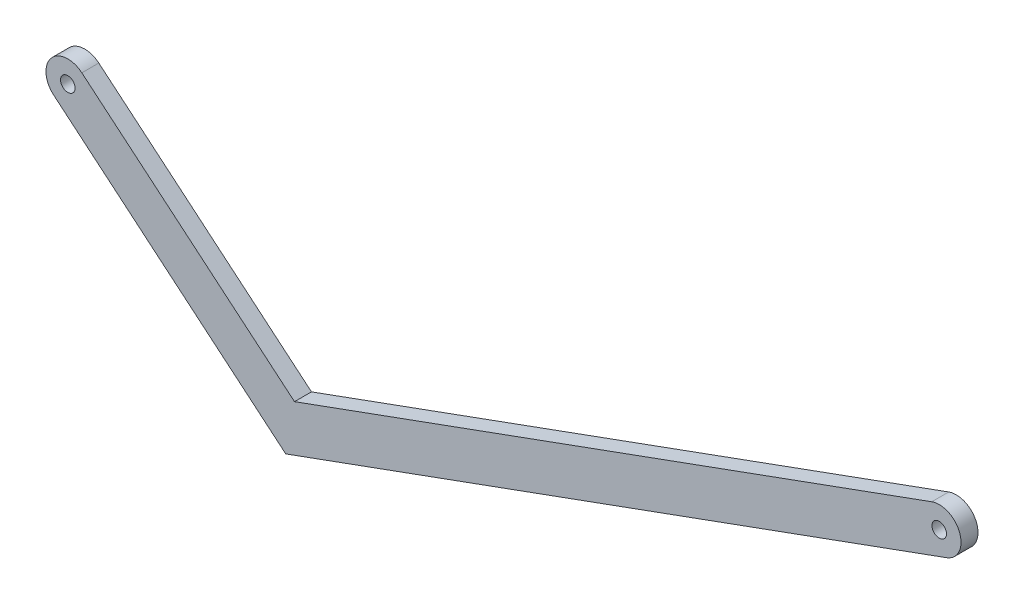
from build123d import *

# Parameters (mm, degrees)
SKETCH_1_R      = 3
EXTRUDE_1_DEPTH = 7


with BuildPart() as part:
    # 草图1 → 凸台-拉伸1 (new body)
    with BuildSketch(Plane.XY):
        with BuildLine():
            Line((362.493953978, 12.044043029), (89.890291348, -87.17557592))
            Line((89.890291348, -87.17557592), (-5.785088487, -6.894399988))
            ThreePointArc((-5.785088487, -6.894399988), (-6.894399988, 5.785088487), (5.785088487, 6.894399988))
            Line((5.785088487, 6.894399988), (93.499500944, -66.706731154))
            Line((93.499500944, -66.706731154), (356.337591398, 28.958510203))
            ThreePointArc((356.337591398, 28.958510203), (367.873006275, 23.579457906), (362.493953978, 12.044043029))
        make_face()
        with Locations((359.415772688, 20.501276616)):
            Circle(SKETCH_1_R, mode=Mode.SUBTRACT)
        Circle(SKETCH_1_R, mode=Mode.SUBTRACT)
    extrude(amount=EXTRUDE_1_DEPTH)


solid = part.part
